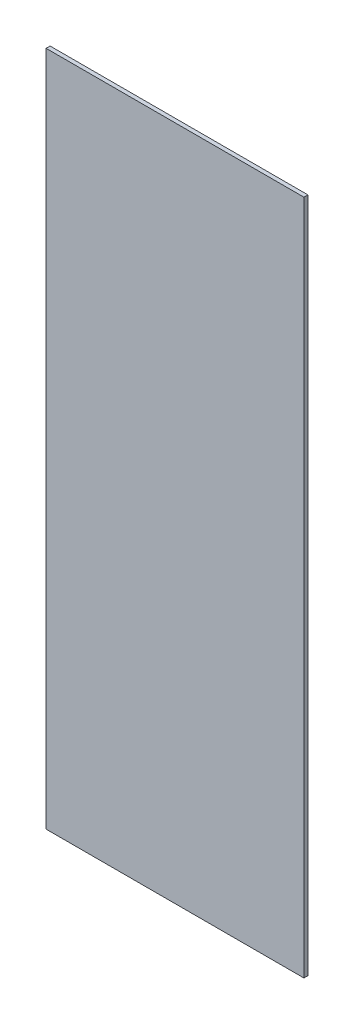
from build123d import *

# Parameters (mm, degrees)
SKETCH_1_W      = 321
SKETCH_1_H      = 842
EXTRUDE_1_DEPTH = 5


with BuildPart() as part:
    # 草图1 → 凸台-拉伸1 (new body)
    with BuildSketch(Plane.XY):
        Rectangle(SKETCH_1_W, SKETCH_1_H)
    extrude(amount=EXTRUDE_1_DEPTH)


solid = part.part
